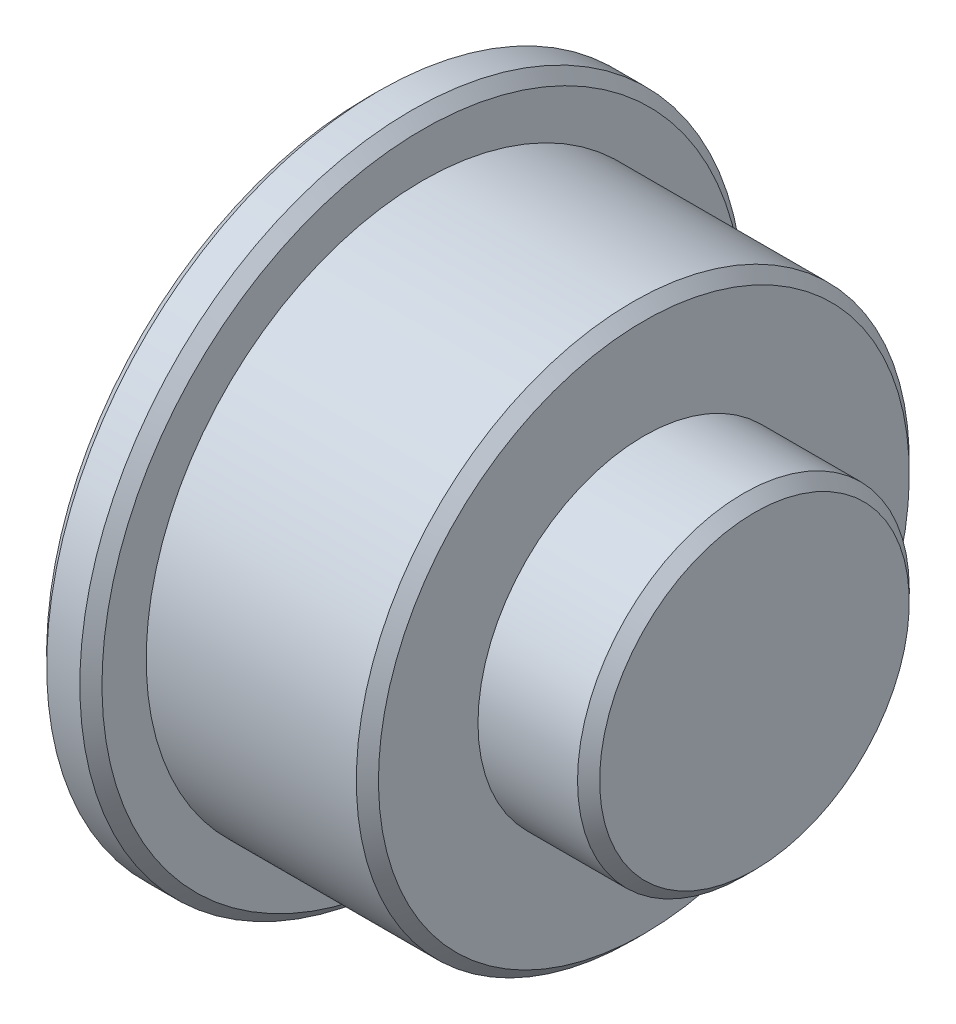
SolidWorks part; units mm, degrees
material "20#"
ref_plane "Front Plane" through (0, 0, 0) normal (0, 0, 1) x (1, 0, 0)
ref_plane "Top Plane" through (0, 0, 0) normal (0, 1, 0) x (1, 0, 0)
ref_plane "Right Plane" through (0, 0, 0) normal (1, 0, 0) x (0, 0, -1)
sketch "Sketch1" plane through (0, 0, 0) normal (0, 0, 1) x (1, 0, 0)
  line L0 (30, 0) -> (-5, 0) construction
  line L1 (30, -15) -> (20, -15)
  line L2 (20, -15) -> (20, -25)
  line L3 (20, -25) -> (0, -25)
  line L4 (0, -25) -> (0, -30)
  line L5 (0, 58) -> (0, -58) construction
  line L6 (0, -30) -> (-5, -30)
  line L7 (-5, -30) -> (-5, 0)
  line L8 (30, -15) -> (30, 0)
  line L9 (-5, 0) -> (30, 0)
  dimension "D1" = 5
  dimension "D2" = 30
  dimension "D3" = 20
  dimension "D4" = 35
  dimension "D5" = 15
  dimension "D6" = 10
revolve "Revolve1" add sketch "Sketch1" angle 360 about L0
chamfer "Chamfer1" distance 1 angle 45 4 edges at (-5, 30, 0) (0, 30, 0) (20, 25, 0) (30, 15, 0)
